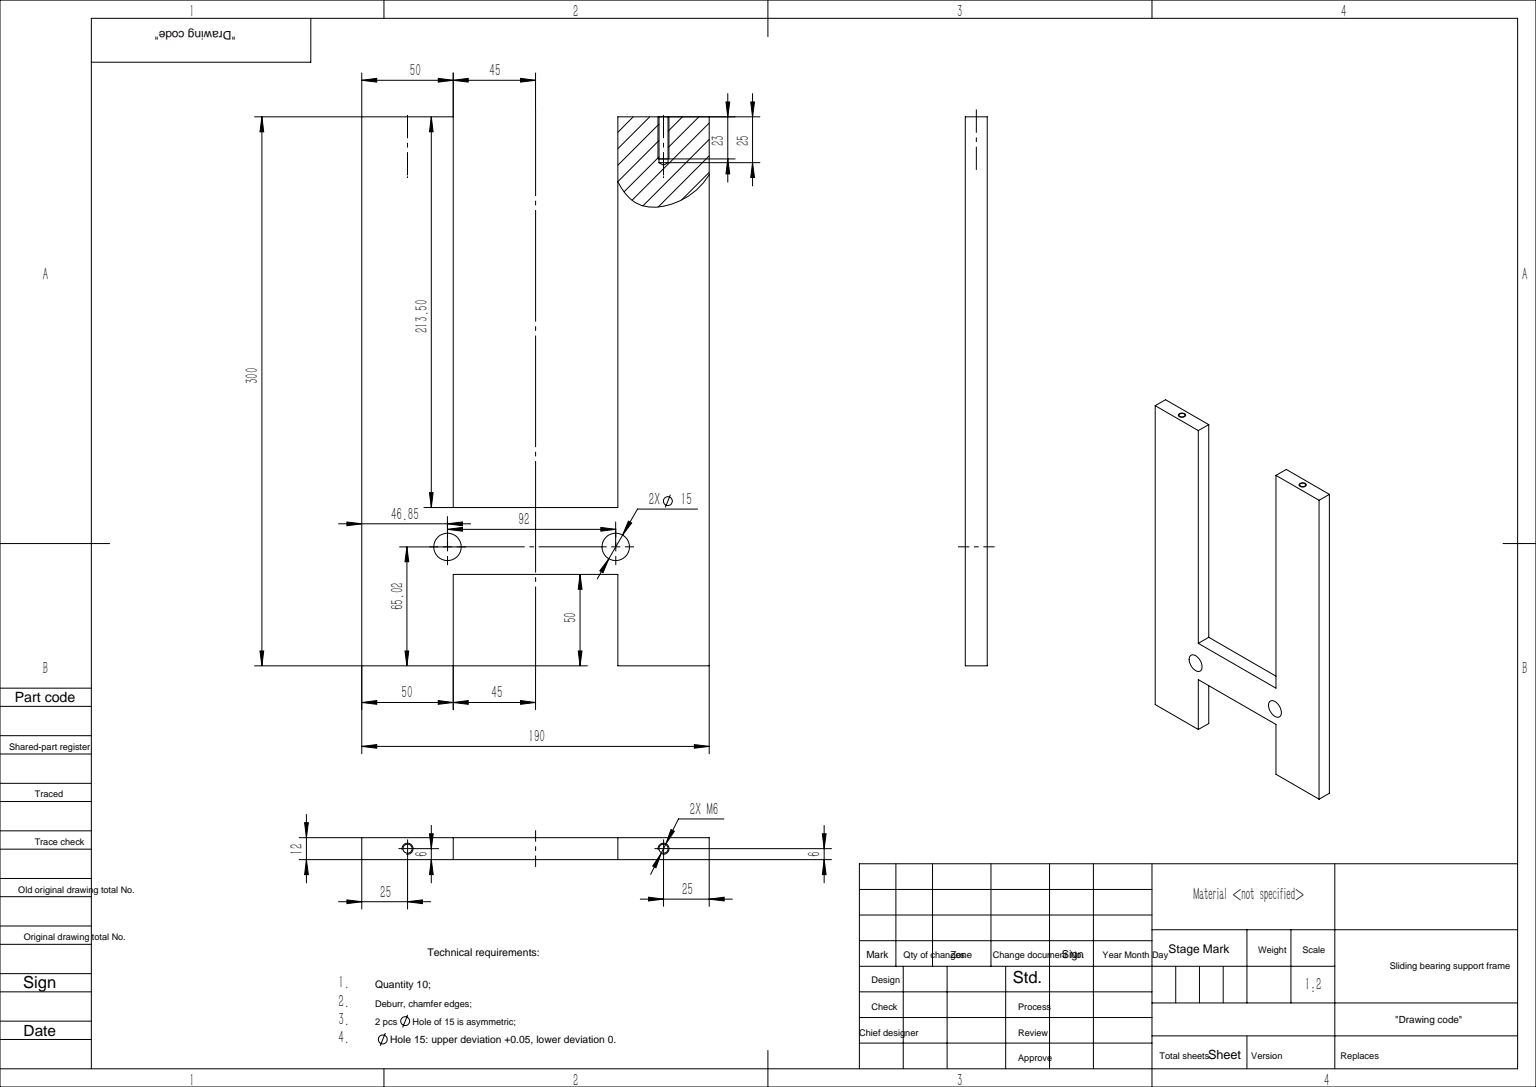
SolidWorks part; units mm, degrees
ref_plane "前视基准面" through (0, 0, 0) normal (0, 0, 1) x (1, 0, 0)
ref_plane "上视基准面" through (0, 0, 0) normal (0, 1, 0) x (1, 0, 0)
ref_plane "右视基准面" through (0, 0, 0) normal (1, 0, 0) x (0, 0, -1)
sketch "草图1" plane through (0, 0, -465) normal (0, 0, -1) x (-1, 0, 0)
  line L0 (-602.0857, 1763.7276) -> (-602.0857, 1440.4628) construction
  line L1 (-557.0857, 1805.0003) -> (-557.0857, 1591.5003)
  line L2 (-557.0857, 1591.5003) -> (-647.0857, 1591.5003)
  line L3 (-557.0857, 1805.0003) -> (-507.0857, 1805.0003)
  line L4 (-507.0857, 1805.0003) -> (-507.0857, 1505.0003)
  line L5 (-507.0857, 1505.0003) -> (-557.0857, 1505.0003)
  line L6 (-647.0857, 1555.0003) -> (-557.0857, 1555.0003)
  line L7 (-557.0857, 1555.0003) -> (-557.0857, 1505.0003)
  line L8 (-557.5857, 1611.0003) -> (-557.5857, 1683.0003) construction
  line L9 (-550.8079, 1611.0003) -> (-565.0497, 1611.0003) construction
  line L10 (-583.6128, 1728.0003) -> (-571.3079, 1728.0003) construction
  line L11 (-647.0857, 1555.0003) -> (-647.0857, 1505.0003)
  line L12 (-697.0857, 1505.0003) -> (-647.0857, 1505.0003)
  line L13 (-647.0857, 1805.0003) -> (-647.0857, 1591.5003)
  line L14 (-697.0857, 1805.0003) -> (-697.0857, 1505.0003)
  line L15 (-647.0857, 1805.0003) -> (-697.0857, 1805.0003)
  circle A0 centre (-553.9391, 1570.019) radius 7.5 construction
  circle A1 centre (-645.9391, 1570.019) radius 7.5 construction
  circle A2 centre (-553.9391, 1570.019) radius 7.5
  circle A3 centre (-645.9391, 1570.019) radius 7.5
  point P18 (-602.0857, 1555.0003)
  point P21 (-602.0857, 1591.5003)
  dimension "D1" = 0.5
  dimension "D2" = 50
  dimension "D3" = 50
  dimension "D4" = 50
  dimension "D5" = 19.5
  dimension "D6" = 77
  dimension "D7" = 300
extrude "凸台-拉伸1" add sketch "草图1" along normal mid plane 12
hole_wizard "M6 螺纹孔1" positions "草图3" profile "草图4" tap size "M6" standard "GB"
sketch "草图3" plane through (0, 1805.0003, 0) normal (0, 1, 0) x (1, 0, 0)
  line L0 (697.0857, 471) -> (697.0857, 459) construction
  line L2 (647.0857, 471) -> (697.0857, 471) construction
  line L3 (602.0857, 432.4586) -> (602.0857, 499.9142) construction
  line L5 (507.0857, 471) -> (507.0857, 459) construction
  point P0 (672.0857, 465)
  point P2 (532.0857, 465)
  point P15 (672.0857, 471)
  dimension "D1" = 25
  dimension "D2" = 6
sketch "草图4" plane through (672.0857, 1805.0003, -465) normal (1, 0, 0) x (0, 0, 1)
  line L0 (0, 0) -> (0, 26.4434)
  line L1 (0, 26.4434) -> (2.5, 25)
  line L2 (2.5, 25) -> (2.5, 0)
  line L5 (2.5, 0) -> (0, 0)
  line L10 (0, 26.4434) -> (-2.5, 25) construction
  line L11 (0, -6.35) -> (0, 107.95) construction
  dimension "螺纹孔钻头直径" = 5
  dimension "螺纹孔钻头深度" = 25
  dimension "导头角度" = 120
cosmetic thread "孔螺蚊线1" parameters "D1"=23, "D2"=6
cosmetic thread "孔螺蚊线2" parameters "D1"=23, "D2"=6
